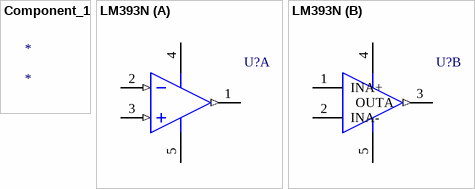
[diagram p0: symbols Component_1 to LM393N]
# Altium schematic symbol library MISC82777-3.SchLib: 2 symbols
Pins are listed as number, name and electrical type; pins without a type are passive.


## Component_1
designator *

## LM393N
designator U?
Dual Comparator
footprint 626-05 (DIP; 8 Leads; Row Spacing 7.62 mm; Pitch 2.54 mm)
3D model 626-05 (DIP; 8 Leads; Row Spacing 7.62 mm; Pitch 2.54 mm)
pins on every part: 4 V+ (power), 5 GND (power)
part A pins: 1 OUT (out), 2 IN- (in), 3 IN+ (in)
part B pins: 1 INA+, 2 INA-, 3 OUTA (out)